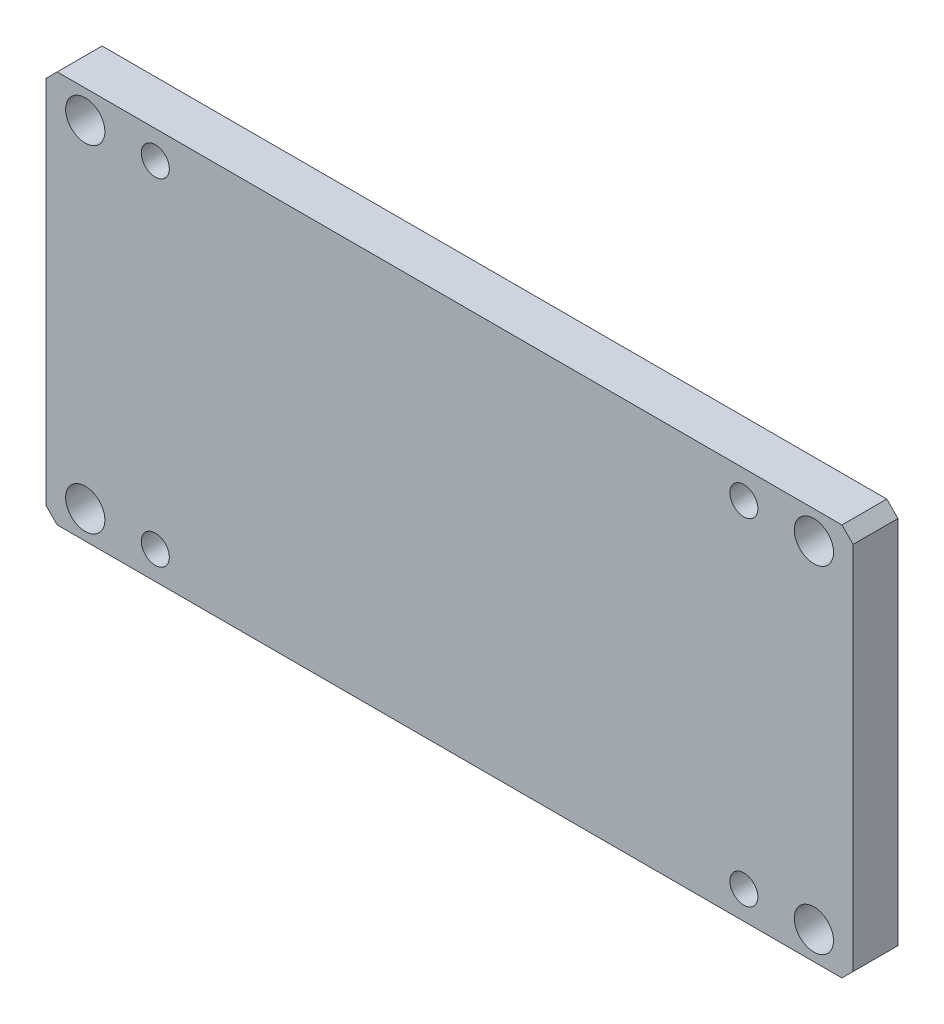
SolidWorks part; units mm, degrees
material "Q235-A"
ref_plane "Front Plane" through (0, 0, 0) normal (0, 0, 1) x (1, 0, 0)
ref_plane "Top Plane" through (0, 0, 0) normal (0, 1, 0) x (1, 0, 0)
ref_plane "Right Plane" through (0, 0, 0) normal (1, 0, 0) x (0, 0, -1)
sketch "Sketch1" plane through (0, 0, 0) normal (0, 0, 1) x (1, 0, 0)
  line L1 (-72, -35) -> (72, -35)
  line L2 (-72, -35) -> (-72, 35)
  line L3 (-72, 35) -> (72, 35)
  line L4 (72, -35) -> (72, 35)
  line L5 (-72, -35) -> (72, 35) construction
  line L6 (-72, 35) -> (72, -35) construction
  line L7 (-65, -30) -> (65, -30) construction
  line L8 (-65, -30) -> (-65, 30) construction
  line L9 (-65, 30) -> (65, 30) construction
  line L10 (65, -30) -> (65, 30) construction
  line L11 (-65, -30) -> (65, 30) construction
  line L12 (-65, 30) -> (65, -30) construction
  circle A0 centre (-65, 30) radius 3.5
  circle A1 centre (-65, -30) radius 3.5
  circle A2 centre (65, -30) radius 3.5
  circle A3 centre (65, 30) radius 3.5
  circle A4 centre (-65, 30) radius 3.5
  point P0 (0, 0)
  point P6 (0, 0)
  dimension "D1" = 144
  dimension "D2" = 70
  dimension "D3" = 60
  dimension "D4" = 130
extrude "Boss-Extrude1" add sketch "Sketch1" along normal blind 8 contours L1 L4 L3 L2 A3 A2 A1 A0
chamfer "Chamfer1" distance 2 angle 45 4 edges at (72, 35, 4) (72, -35, 4) (-72, -35, 4) (-72, 35, 4)
sketch "Sketch2" plane through (0, 0, 8) normal (0, 0, 1) x (1, 0, 0)
  line L1 (-52.5, -30) -> (52.5, -30)
  line L2 (-52.5, -30) -> (-52.5, 30)
  line L3 (-52.5, 30) -> (52.5, 30)
  line L4 (52.5, -30) -> (52.5, 30)
  line L5 (-52.5, -30) -> (52.5, 30) construction
  line L6 (-52.5, 30) -> (52.5, -30) construction
  point P0 (0, 0)
  dimension "D1" = 60
  dimension "D2" = 105
hole_wizard "M6 Tapped Hole1" positions "Sketch3" profile "Sketch4" tap size "M6" standard "GB" end condition through all
sketch "Sketch3" plane through (0, 0, 8) normal (0, 0, 1) x (1, 0, 0)
  point P0 (-52.5, 30)
  point P3 (-52.5, -30)
  point P6 (52.5, -30)
  point P9 (52.5, 30)
sketch "Sketch4" plane through (-52.5, 30, 8) normal (1, 0, 0) x (0, -1, 0)
  line L0 (0, 0) -> (0, 8)
  line L1 (0, 8) -> (2.5, 8)
  line L2 (2.5, 8) -> (2.5, 0)
  line L5 (2.5, 0) -> (0, 0)
  line L11 (0, -6.35) -> (0, 107.95) construction
  dimension "通孔螺纹孔钻头直径" = 5
  dimension "通孔螺纹孔钻头深度" = 8
cosmetic thread "Cosmetic Thread1" parameters "D2"=6
cosmetic thread "Cosmetic Thread2" parameters "D2"=6
cosmetic thread "Cosmetic Thread3" parameters "D2"=6
cosmetic thread "Cosmetic Thread4" parameters "D2"=6
